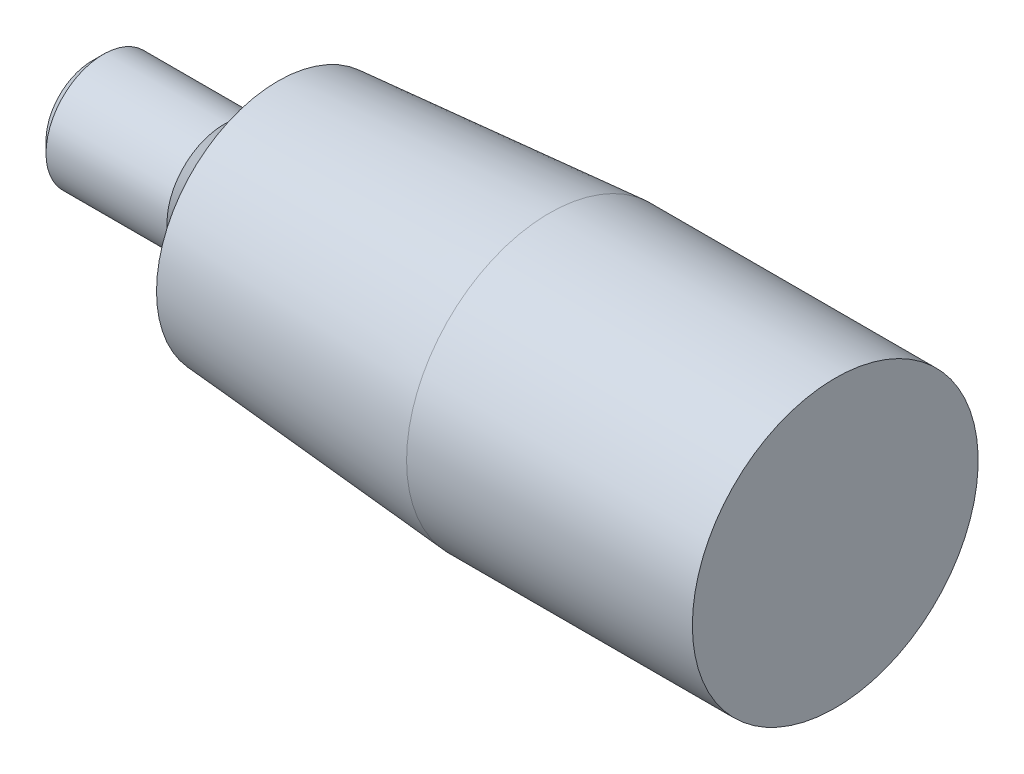
from build123d import *

# Parameters (mm, degrees)
CUT_EXTRUDE1_DEPTH = 4


with BuildPart() as part:
    # Sketch1 → Revolve1 (revolve)
    with BuildSketch(Plane.XY, mode=Mode.PRIVATE) as revolve1_sk:
        Polygon((-13, 0), (-13, 3.233), (-12.233, 4), (-3.767, 4), (-3.0905, 3.3235), (-1, 3.3235), (-1, 5), (0, 5), (0, 8.5), (19, 10), (39, 10), (39, 0), align=None)
    revolve(revolve1_sk.sketch.rotate(Axis((39, 0, 0), (-1, 0, 0)), 270), axis=Axis((39, 0, 0), (-1, 0, 0)))

    # Sketch2 → Cut-Extrude1 (cut)
    with BuildSketch(Plane(origin=(-13, 0, 0), x_dir=(0, 0, -1), z_dir=(1, 0, 0))):
        Polygon((-2, 1.154700538), (-2, -1.154700538), (0, -2.309401077), (2, -1.154700538), (2, 1.154700538), (0, 2.309401077), align=None)
    extrude(amount=CUT_EXTRUDE1_DEPTH, mode=Mode.SUBTRACT)

    # Sketch3 → Cut-Revolve1 (revolve, cut)
    with BuildSketch(Plane.XY, mode=Mode.PRIVATE) as cut_revolve1_sk:
        Polygon((-9, 0), (-9, 2.309401077), (-7.67, 0), align=None)
    revolve(cut_revolve1_sk.sketch.rotate(Axis((-7.67, 0, 0), (-1, 0, 0)), 270), axis=Axis((-7.67, 0, 0), (-1, 0, 0)), mode=Mode.SUBTRACT)


solid = part.part
